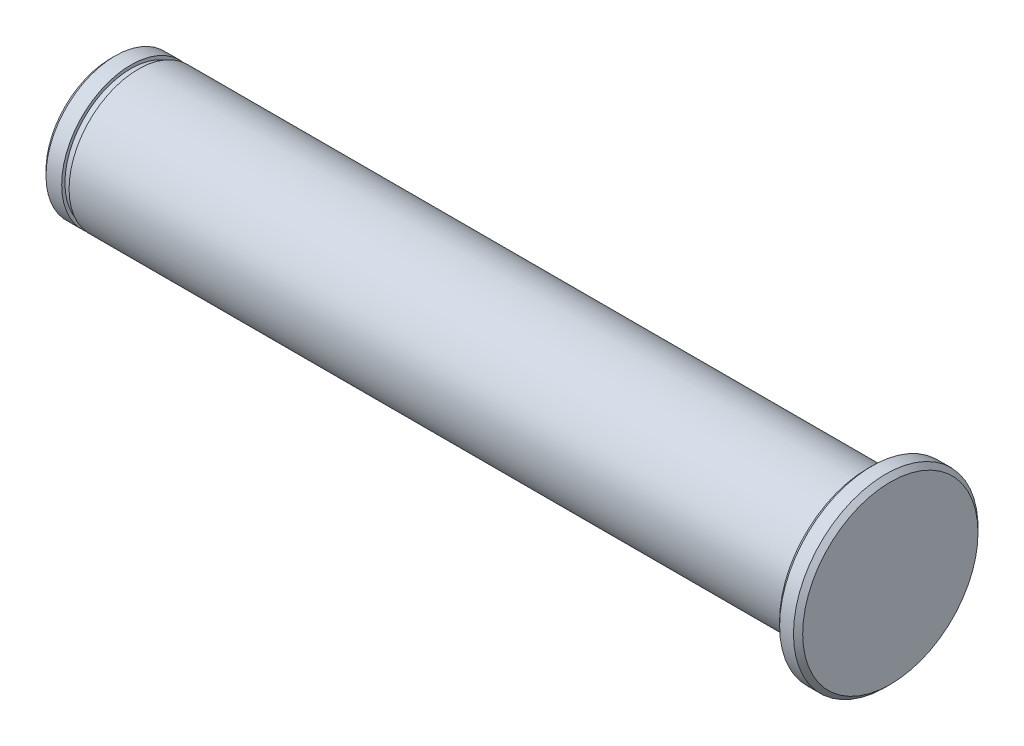
SolidWorks part; units mm, degrees
material "45#"
ref_plane "前基準面" through (0, 0, 0) normal (0, 0, 1) x (1, 0, 0)
ref_plane "上基準面" through (0, 0, 0) normal (0, 1, 0) x (1, 0, 0)
ref_plane "右基準面" through (0, 0, 0) normal (1, 0, 0) x (0, 0, -1)
sketch "草图1" plane through (0, 0, 0) normal (0, 0, 1) x (1, 0, 0)
  line L0 (0, 0) -> (172.6747, 0) construction
  line L3 (0, 0) -> (0, 15)
  line L6 (0, 15) -> (4.4, 15)
  line L7 (164, 15) -> (164, 20)
  line L8 (164, 20) -> (169, 20)
  line L9 (169, 20) -> (169, 0)
  line L12 (169, 0) -> (0, 0)
  line L15 (4.4, 15) -> (4.4, 14.3)
  line L16 (4.4, 14.3) -> (6, 14.3)
  line L17 (6, 14.3) -> (6, 15)
  line L18 (6, 15) -> (164, 15)
  dimension "D2" = 30
  dimension "D3" = 164
  dimension "D4" = 40
  dimension "D7" = 1.6
  dimension "D8" = 5
  dimension "D9" = 28.6
  dimension "D10" = 6
  dimension "D11" = 4.4
revolve "旋转1" add sketch "草图1" angle 360 about L0
sketch "草图2" plane through (0, 0, 0) normal (0, 0, 1) x (1, 0, 0)
  line L0 (0, 0) -> (179.0245, 0) construction
  line L1 (0, 15) -> (0, -15) construction
  line L2 (119, 0) -> (49, 0) construction
  line L3 (119, -4) -> (49, -4)
  line L4 (119, 4) -> (49, 4)
  line L5 (164, 15) -> (164, -15) construction
  arc A0 (119, -4) -> (119, 4) centre (119, 0) ccw
  arc A1 (49, 4) -> (49, -4) centre (49, 0) ccw
  point P6 (84, 0)
  dimension "D1" = 4
  dimension "D2" = 80
  dimension "D3" = 70
extrude "切除-拉伸1" cut sketch "草图2" along normal blind 4 from offset 15 offset against normal yes
chamfer "倒角1" distance 1 angle 45 3 edges at (164, 0, 20) (169, 0, 20) (0, 0, 15)
